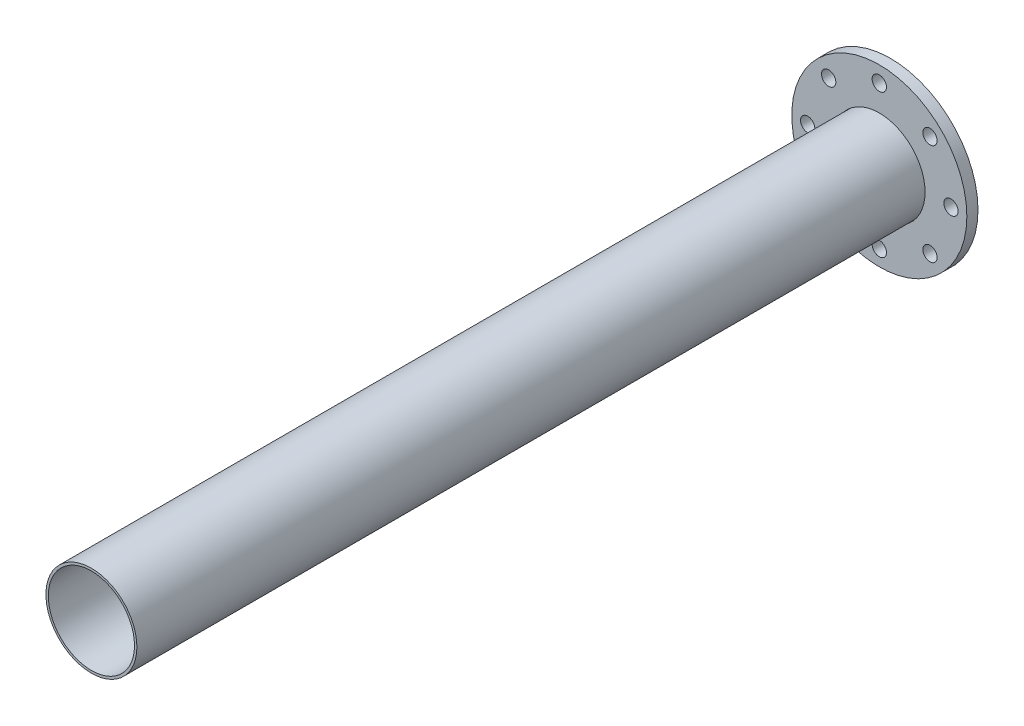
SolidWorks part; units mm, degrees
material "Plain carbon steel"
ref_plane "Front Plane" through (0, 0, 0) normal (0, 0, 1) x (1, 0, 0)
ref_plane "Top Plane" through (0, 0, 0) normal (0, 1, 0) x (1, 0, 0)
ref_plane "Right Plane" through (0, 0, 0) normal (1, 0, 0) x (0, 0, -1)
sketch "Sketch1" plane through (0, 0, 0) normal (0, 0, 1) x (1, 0, 0)
  circle A0 centre (0, 0) radius 110
  circle A1 centre (0, 0) radius 90 construction
  circle A2 centre (0, 0) radius 57.5
  circle A3 centre (0, 90) radius 9
  circle A4 centre (63.6396, 63.6396) radius 9
  circle A5 centre (90, 0) radius 9
  circle A6 centre (63.6396, -63.6396) radius 9
  circle A7 centre (0, -90) radius 9
  circle A8 centre (-63.6396, -63.6396) radius 9
  circle A9 centre (-90, 0) radius 9
  circle A10 centre (-63.6396, 63.6396) radius 9
  dimension "D1" = 115
  dimension "D2" = 180
  dimension "D3" = 220
  dimension "D4" = 18
  dimension "D5" = 8
extrude "Boss-Extrude1" add sketch "Sketch1" along normal blind 14
ref_plane "Plane1" through (0, 0, 4) normal (0, 0, 1) x (1, 0, 0)
sketch "Sketch2" plane through (0, 0, 4) normal (0, 0, 1) x (1, 0, 0)
  circle A0 centre (0, 0) radius 57.15
  circle A1 centre (0, 0) radius 54.15
  dimension "D1" = 114.3
  dimension "D2" = 3
extrude "Boss-Extrude2" add sketch "Sketch2" along normal blind 1000 separate body
